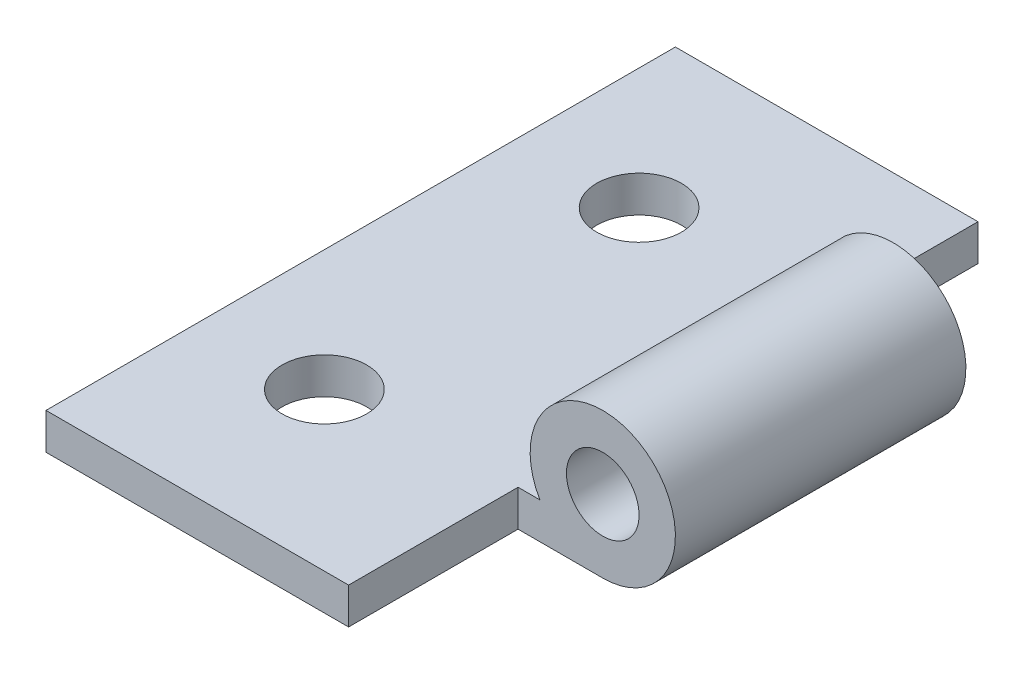
SolidWorks part; units mm, degrees
material "AISI 304"
ref_plane "前视基准面" through (0, 0, 0) normal (0, 0, 1) x (1, 0, 0)
ref_plane "上视基准面" through (0, 0, 0) normal (0, 1, 0) x (1, 0, 0)
ref_plane "右视基准面" through (0, 0, 0) normal (1, 0, 0) x (0, 0, -1)
sketch "草图1" plane through (0, 0, 0) normal (0, 0, 1) x (1, 0, 0)
  line L0 (-2.5981, -1.5) -> (-16, -1.5)
  line L1 (-16, -1.5) -> (-16, -3)
  line L2 (-16, -3) -> (0, -3)
  circle A0 centre (0, 0) radius 1.5
  arc A1 (0, -3) -> (-2.5981, -1.5) centre (0, 0) ccw
  dimension "D1" = 6
  dimension "D2" = 3
  dimension "D3" = 16
extrude "凸台-拉伸1" add sketch "草图1" along normal mid plane 26
sketch "草图2" plane through (0, 0, 13) normal (0, 0, 1) x (1, 0, 0)
  line L0 (-3.5, 0) -> (-3.5, -3)
  line L1 (-16, -3) -> (0, -3) construction
  line L3 (-3.5, -3) -> (-1.8028, -3)
  arc A0 (-1.8028, -3) -> (-3.5, 0) centre (0, 0) ccw
  dimension "D1" = 3.5
extrude "切除-拉伸3" cut sketch "草图2" against normal blind 7
sketch "草图4" plane through (0, 0, -13) normal (0, 0, -1) x (-1, 0, 0)
  line L2 (3.5, -3) -> (3.5, 0)
  line L3 (1.8028, -3) -> (3.5, -3)
  line L4 (3.5, -3) -> (3.5, 0)
  line L5 (1.8028, -3) -> (3.5, -3)
  arc A1 (3.5, 0) -> (1.8028, -3) centre (0, 0) ccw
  arc A2 (3.5, 0) -> (1.8028, -3) centre (0, 0) ccw
  dimension "D1" = 0
extrude "切除-拉伸4" cut sketch "草图4" against normal blind 7
sketch "草图3" plane through (0, -1.5, 0) normal (0, 1, 0) x (1, 0, 0)
  line L0 (0, 0) -> (-16, 0) construction
  line L1 (-16, -13) -> (-16, 13) construction
  circle A0 centre (-11, 6.5) radius 1.75
  circle A1 centre (-11, -6.5) radius 1.75
  dimension "D1" = 3.5
  dimension "D2" = 11
  dimension "D3" = 13
extrude "切除-拉伸2" cut sketch "草图3" against normal through all
